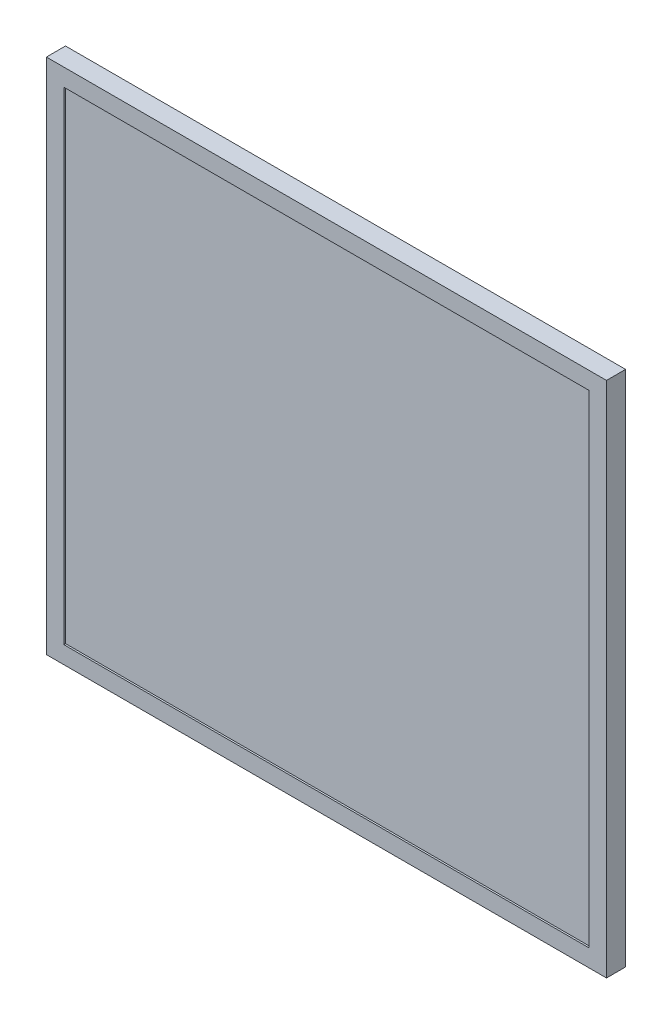
SolidWorks part; units mm, degrees
ref_plane "前视基准面" through (0, 0, 0) normal (0, 0, 1) x (1, 0, 0)
ref_plane "上视基准面" through (0, 0, 0) normal (0, 1, 0) x (1, 0, 0)
ref_plane "右视基准面" through (0, 0, 0) normal (1, 0, 0) x (0, 0, -1)
sketch "草图1" plane through (0, 0, 0) normal (0, 0, 1) x (1, 0, 0)
  line L1 (0, 0) -> (645, 0)
  line L2 (0, 0) -> (0, 596)
  line L3 (0, 596) -> (645, 596)
  line L4 (645, 0) -> (645, 596)
  dimension "D1" = 596
  dimension "D2" = 645
extrude "凸台-拉伸1" add sketch "草图1" along normal blind 22
shell "抽壳1" thickness 2
sketch "草图2" plane through (0, 0, 22) normal (0, 0, 1) x (1, 0, 0)
  line L14 (20, 576) -> (20, 20)
  line L15 (20, 20) -> (625, 20)
  line L16 (625, 20) -> (625, 576)
  line L17 (625, 576) -> (20, 576)
  line L18 (20, 576) -> (20, 20)
  line L19 (20, 20) -> (625, 20)
  line L20 (625, 20) -> (625, 576)
  line L21 (625, 576) -> (20, 576)
  line L26 (0, 596) -> (0, 0)
  line L27 (0, 0) -> (645, 0)
  line L28 (645, 0) -> (645, 596)
  line L29 (645, 596) -> (0, 596)
  line L30 (0, 596) -> (0, 0)
  line L31 (0, 0) -> (645, 0)
  line L32 (645, 0) -> (645, 596)
  line L33 (645, 596) -> (0, 596)
  dimension "D1" = 20
  dimension "D2" = 0
extrude "凸台-拉伸2" add sketch "草图2" against normal blind 2
